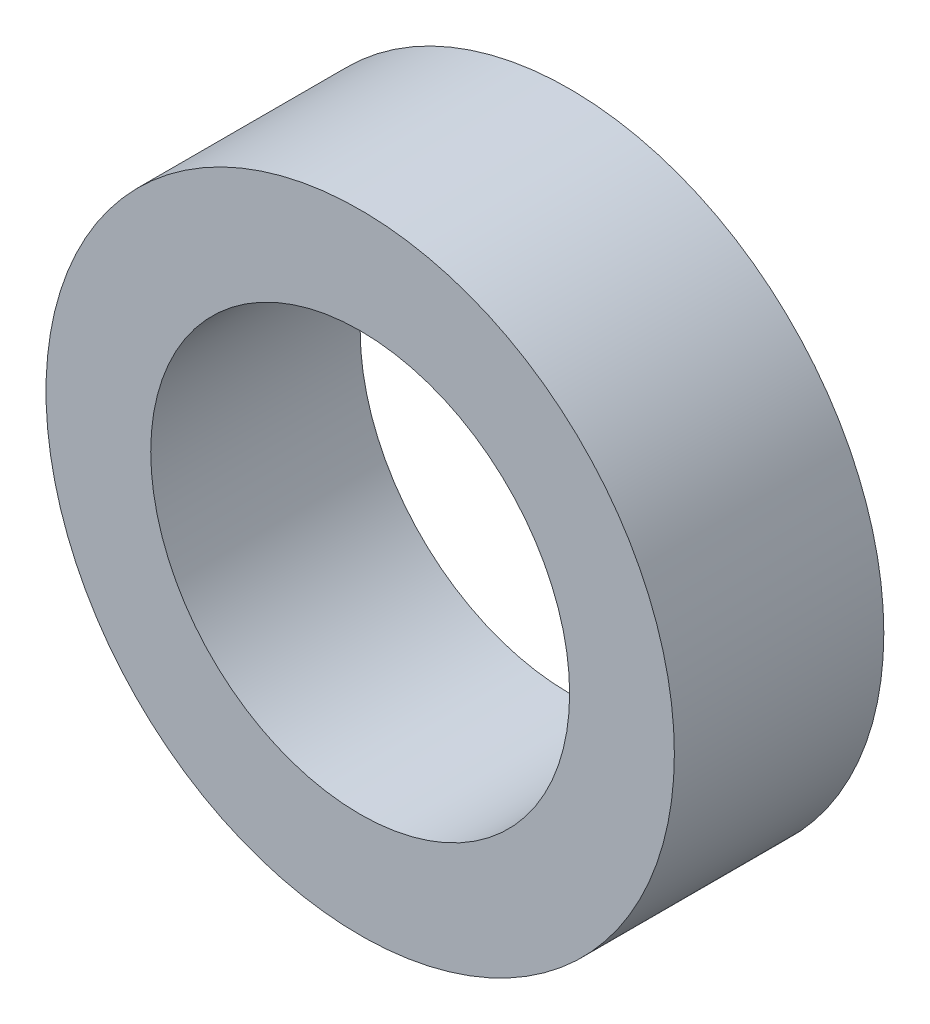
from build123d import *

# Parameters (mm, degrees)
SKETCH1_R           = 3
SKETCH1_R_2         = 2
BOSS_EXTRUDE1_DEPTH = 2


with BuildPart() as part:
    # Sketch1 → Boss-Extrude1 (new body)
    with BuildSketch(Plane.XY):
        Circle(SKETCH1_R)
        Circle(SKETCH1_R_2, mode=Mode.SUBTRACT)
    extrude(amount=BOSS_EXTRUDE1_DEPTH)


solid = part.part
